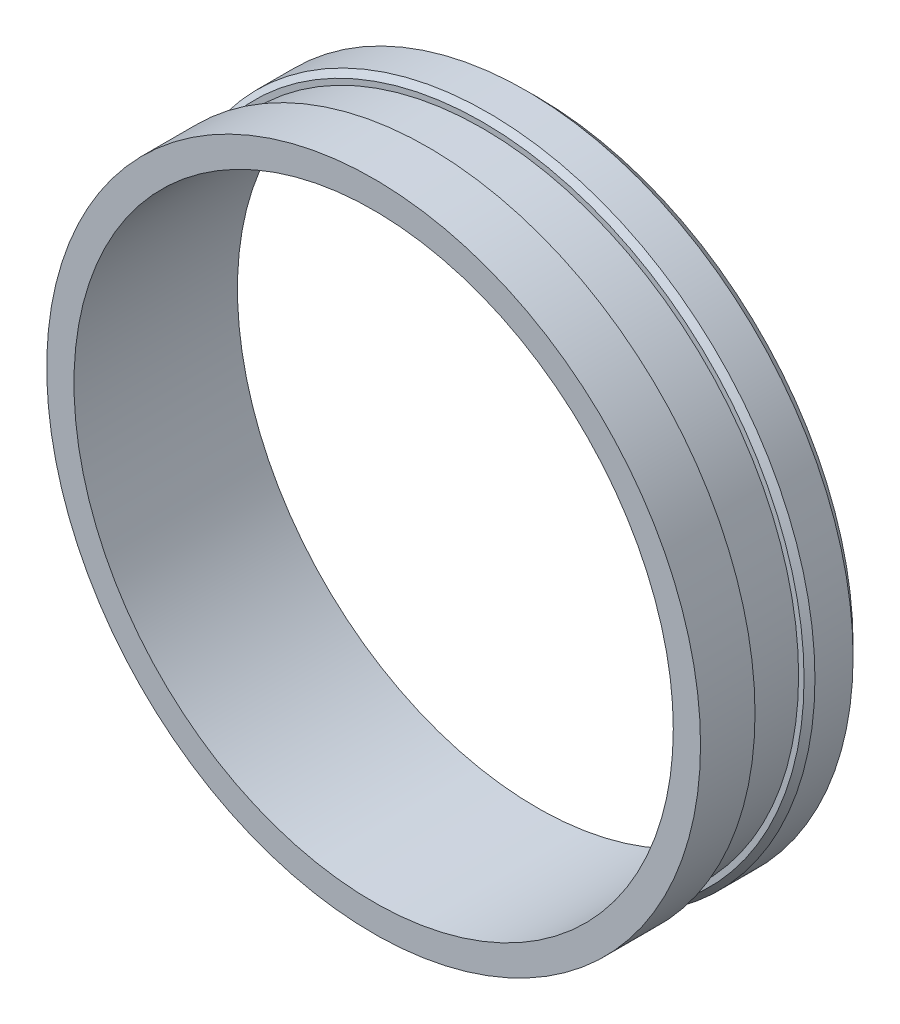
from build123d import *

# Parameters (mm, degrees)
SKETCH1_R           = 60
SKETCH1_R_2         = 55
BOSS_EXTRUDE1_DEPTH = 20
CUT_EXTRUDE1_START  = -10
SKETCH2_R           = 60
SKETCH2_R_2         = 58
CUT_EXTRUDE1_DEPTH  = 10
SKETCH3_R           = 60
SKETCH3_R_2         = 55
BOSS_EXTRUDE2_DEPTH = 10
CHAMFER1_SIZE       = 2
CHAMFER2_SIZE       = 1


with BuildPart() as part:
    # Sketch1 → Boss-Extrude1 (new body)
    with BuildSketch(Plane.XY):
        Circle(SKETCH1_R)
        Circle(SKETCH1_R_2, mode=Mode.SUBTRACT)
    extrude(amount=BOSS_EXTRUDE1_DEPTH)

    # Sketch2 → Cut-Extrude1 (cut)
    with BuildSketch(Plane.XY.offset(20).offset(CUT_EXTRUDE1_START)):
        Circle(SKETCH2_R)
        Circle(SKETCH2_R_2, mode=Mode.SUBTRACT)
    extrude(amount=CUT_EXTRUDE1_DEPTH, mode=Mode.SUBTRACT)

    # Sketch3 → Boss-Extrude2 (add)
    with BuildSketch(Plane.XY.offset(20)):
        Circle(SKETCH3_R)
        Circle(SKETCH3_R_2, mode=Mode.SUBTRACT)
    extrude(amount=BOSS_EXTRUDE2_DEPTH)

    # Chamfer1
    chamfer1_edges = [part.edges().sort_by_distance(p)[0] for p in [
        (-60, 0, 0),
    ]]
    chamfer(chamfer1_edges, length=CHAMFER1_SIZE)

    # Chamfer2
    chamfer2_edges = [part.edges().sort_by_distance(p)[0] for p in [
        (-60, 0, 10),
    ]]
    chamfer(chamfer2_edges, length=CHAMFER2_SIZE)


solid = part.part
